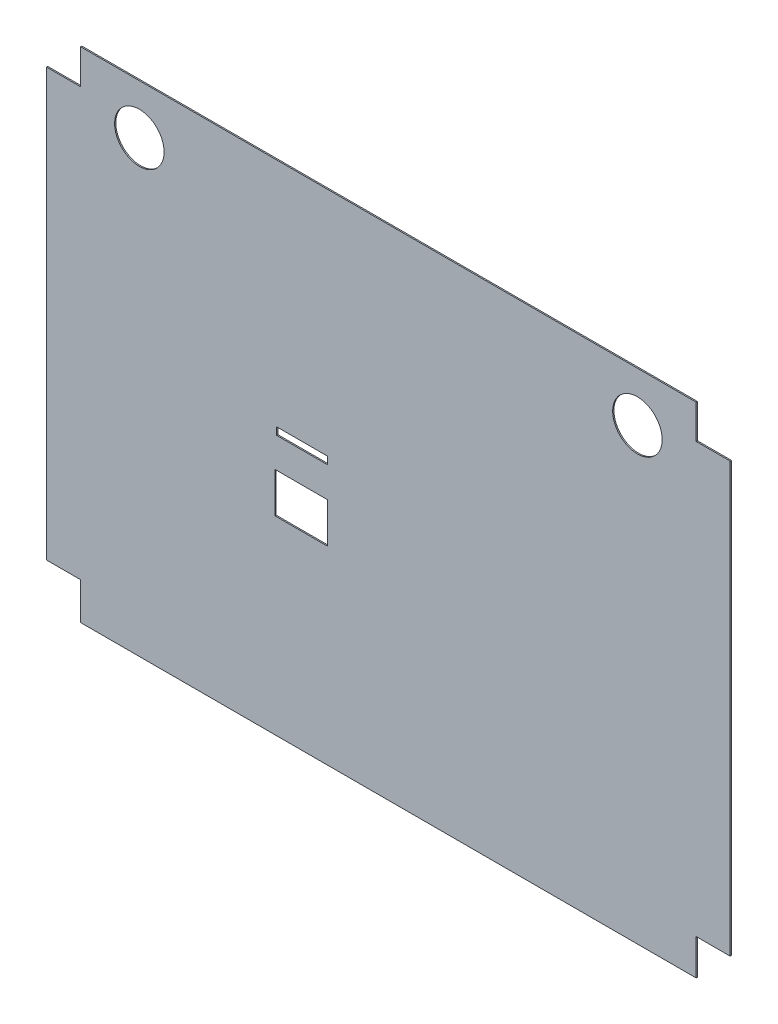
SolidWorks part; units mm, degrees
ref_plane "前视基准面" through (0, 0, 0) normal (0, 0, 1) x (1, 0, 0)
ref_plane "上视基准面" through (0, 0, 0) normal (0, 1, 0) x (1, 0, 0)
ref_plane "右视基准面" through (0, 0, 0) normal (1, 0, 0) x (0, 0, -1)
sketch "草图1" plane through (0, 0, 0) normal (0, 0, 1) x (1, 0, 0)
  line L0 (-367.7707, 104.2338) -> (-312.7707, 104.2338)
  line L1 (-312.7707, 160.2338) -> (682.2293, 160.2338)
  line L2 (-367.7707, 104.2338) -> (-367.7707, -585.7662)
  line L3 (-312.7707, -645.7662) -> (682.2293, -645.7662)
  line L4 (737.2293, 105.2338) -> (737.2293, -587.7662)
  line L5 (-312.7707, 104.2338) -> (-312.7707, 160.2338)
  line L6 (-367.7707, -585.7662) -> (-312.7707, -585.7662)
  line L7 (-312.7707, -585.7662) -> (-312.7707, -645.7662)
  line L8 (737.2293, -587.7662) -> (682.2293, -587.7662)
  line L9 (682.2293, -587.7662) -> (682.2293, -645.7662)
  line L10 (737.2293, 105.2338) -> (682.2293, 105.2338)
  line L11 (682.2293, 105.2338) -> (682.2293, 160.2338)
  circle A0 centre (-217.7707, 80.2338) radius 40
  circle A1 centre (587.2293, 80.2338) radius 40
  dimension "D13" = 80
  dimension "D16" = 80
  dimension "D2" = 995
  dimension "D3" = 56
  dimension "D4" = 55
  dimension "D5" = 55
  dimension "D6" = 60
  dimension "D7" = 58
  dimension "D8" = 55
  dimension "D9" = 55
  dimension "D10" = 55
  dimension "D11" = 150
  dimension "D12" = 80
  dimension "D14" = 150
  dimension "D15" = 80
  dimension "D17" = 690
extrude "凸台-拉伸1" add sketch "草图1" along normal blind 2
extrude "切除-拉伸2" cut sketch "草图3" against normal blind 2
sketch "草图3" plane through (995.4355, 654.4533, 0) normal (0, 0, -1) x (0, -1, 0)
  line L0 (867.744, 991.1439) -> (867.744, 909.1439)
  line L1 (867.744, 909.1439) -> (879.744, 909.1439)
  line L2 (879.744, 909.1439) -> (879.744, 991.1439)
  line L3 (879.744, 991.1439) -> (867.744, 991.1439)
extrude "切除-拉伸3" cut sketch "草图4" against normal up to surface (2 mm away) up to face at (45.2916, -219.2907, 2)
sketch "草图4" plane through (995.4355, 654.4533, 0) normal (0, 0, -1) x (0, -1, 0)
  line L0 (928.744, 949.1439) -> (928.744, 909.1439)
  line L1 (928.744, 994.1439) -> (993.744, 994.1439)
  line L2 (928.744, 994.1439) -> (928.744, 949.1439)
  line L4 (993.744, 994.1439) -> (993.744, 949.1439)
  line L5 (928.744, 909.1439) -> (993.744, 909.1439)
  line L6 (993.744, 909.1439) -> (993.744, 949.1439)
